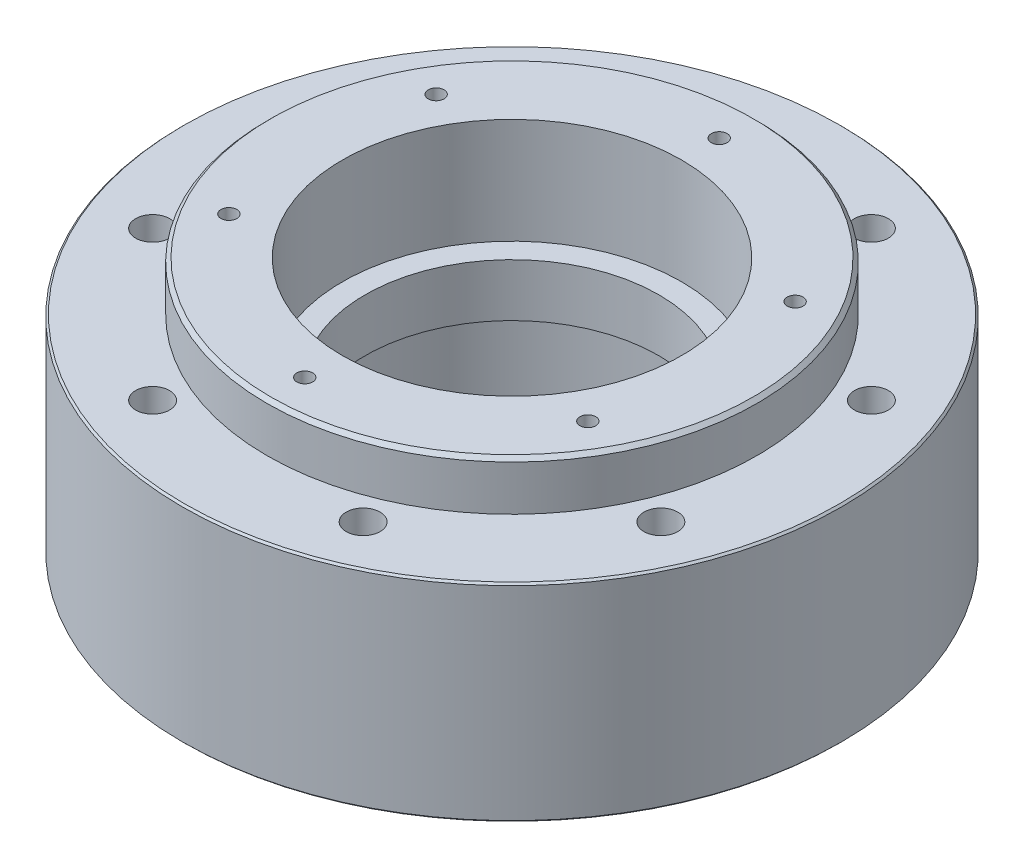
from build123d import *

# Parameters (mm, degrees)
SKETCH1_R                                          = 87.5
BOSS_EXTRUDE1_DEPTH                                = 55
SKETCH2_R                                          = 65
BOSS_EXTRUDE2_DEPTH                                = 13
SKETCH3_R                                          = 57.5
BOSS_EXTRUDE3_DEPTH                                = 5
SKETCH4_R                                          = 45
CUT_EXTRUDE1_DEPTH                                 = 31
CUT_EXTRUDE2_START                                 = -28
SKETCH5_R                                          = 45
CUT_EXTRUDE2_DEPTH                                 = 28
SKETCH6_R                                          = 39
CUT_EXTRUDE3_DEPTH                                 = 132.671940823
CHAMFER1_SIZE                                      = 1
HOLE_SIZE_BASED_ON_SOCKET_HEAD_CAP_SCR_D           = 9
HOLE_SIZE_BASED_ON_SOCKET_HEAD_CAP_SCR_CBORE_D     = 15
HOLE_SIZE_BASED_ON_SOCKET_HEAD_CAP_SCR_CBORE_DEPTH = 30
CIRPATTERN1_COUNT                                  = 8
CHAMFER2_SIZE                                      = 0.5
CIRPATTERN2_COUNT                                  = 8
CIRPATTERN3_COUNT                                  = 6


with BuildPart() as part:
    # Sketch1 → Boss-Extrude1 (new body)
    with BuildSketch(Plane(origin=(0, 0, 0), x_dir=(1, 0, 0), z_dir=(0, 1, 0))):
        with Locations(Location((0, 0, 0), (0, 0, 270))):
            Circle(SKETCH1_R)
    extrude(amount=BOSS_EXTRUDE1_DEPTH)

    # Sketch2 → Boss-Extrude2 (add)
    with BuildSketch(Plane(origin=(0, 55, 0), x_dir=(1, 0, 0), z_dir=(0, 1, 0))):
        with Locations(Location((0, 0, 0), (0, 0, 270))):
            Circle(SKETCH2_R)
    extrude(amount=BOSS_EXTRUDE2_DEPTH)

    # Sketch3 → Boss-Extrude3 (add)
    with BuildSketch(Plane.XZ):
        with Locations(Location((0, 0, 0), (0, 0, 90))):
            Circle(SKETCH3_R)
    extrude(amount=BOSS_EXTRUDE3_DEPTH)

    # Sketch4 → Cut-Extrude1 (cut)
    with BuildSketch(Plane.XZ.offset(5)):
        with Locations(Location((0, 0, 0), (0, 0, 270))):
            Circle(SKETCH4_R)
    extrude(amount=-CUT_EXTRUDE1_DEPTH, mode=Mode.SUBTRACT)

    # Sketch5 → Cut-Extrude2 (cut)
    with BuildSketch(Plane(origin=(0, 68, 0), x_dir=(1, 0, 0), z_dir=(0, 1, 0)).offset(CUT_EXTRUDE2_START)):
        with Locations(Location((0, 0, 0), (0, 0, 90))):
            Circle(SKETCH5_R)
    extrude(amount=CUT_EXTRUDE2_DEPTH, mode=Mode.SUBTRACT)

    # Sketch6 → Cut-Extrude3 (cut, through all)
    with BuildSketch(Plane(origin=(0, 40, 0), x_dir=(1, 0, 0), z_dir=(0, 1, 0))):
        with Locations(Location((0, 0, 0), (0, 0, 270))):
            Circle(SKETCH6_R)
    extrude(amount=-CUT_EXTRUDE3_DEPTH, mode=Mode.SUBTRACT)

    # Chamfer1
    chamfer1_edges = [part.edges().sort_by_distance(p)[0] for p in [
        (0, -5, -57.5),
        (0, 68, -65),
    ]]
    chamfer(chamfer1_edges, length=CHAMFER1_SIZE)

    # Hole size (% based on socket head cap screw type)1 (through all)
    with Locations(Plane(origin=(0, 0, 0), x_dir=(-1, 0, 0), z_dir=(0, -1, 0))):
        with Locations((-67.443205873, 27.935890563)):
            hole_size_based_on_socket_head_cap_scr = CounterBoreHole(HOLE_SIZE_BASED_ON_SOCKET_HEAD_CAP_SCR_D / 2, HOLE_SIZE_BASED_ON_SOCKET_HEAD_CAP_SCR_CBORE_D / 2, HOLE_SIZE_BASED_ON_SOCKET_HEAD_CAP_SCR_CBORE_DEPTH)

    # CirPattern1: Hole size (% based on socket head cap screw type)1 ×8 about axis
    cirpattern1_axis = Axis((0, 0, 0), (0, 1, 0))
    for i in range(1, CIRPATTERN1_COUNT):
        add(hole_size_based_on_socket_head_cap_scr.rotate(cirpattern1_axis, i * 360 / CIRPATTERN1_COUNT), mode=Mode.SUBTRACT)

    # Chamfer2
    chamfer2_edges = [part.edges().sort_by_distance(p)[0] for p in [
        (0, 0, -87.5),
        (0, 55, -87.5),
    ]]
    chamfer(chamfer2_edges, length=CHAMFER2_SIZE)

    # Sketch13 → M10 Tapped Hole1 (revolve, cut)
    with BuildSketch(Plane(origin=(0, 0, -67.5), x_dir=(0, 0, -1), z_dir=(1, 0, 0))):
        Polygon((0, 0), (0, 40.053657631), (4.25, 37.5), (4.25, 0), align=None)
    m10_tapped_hole1 = revolve(axis=Axis((0, -6.35, -67.5), (0, 1, 0)), mode=Mode.SUBTRACT)

    # CirPattern2: M10 Tapped Hole1 ×8 about axis
    cirpattern2_axis = Axis((0, 0, 0), (0, 1, 0))
    for i in range(1, CIRPATTERN2_COUNT):
        add(m10_tapped_hole1.rotate(cirpattern2_axis, i * 360 / CIRPATTERN2_COUNT), mode=Mode.SUBTRACT)

    # Sketch15 → M5 Tapped Hole1 (revolve, cut)
    with BuildSketch(Plane(origin=(0, 68, 55), x_dir=(0, 0, 1), z_dir=(1, 0, 0))):
        Polygon((0, 0), (0, 15.2618073), (2.1, 14), (2.1, 0), align=None)
    m5_tapped_hole1 = revolve(axis=Axis((0, 74.35, 55), (0, -1, 0)), mode=Mode.SUBTRACT)

    # CirPattern3: M5 Tapped Hole1 ×6 about axis
    cirpattern3_axis = Axis((0, 0, 0), (0, 1, 0))
    for i in range(1, CIRPATTERN3_COUNT):
        add(m5_tapped_hole1.rotate(cirpattern3_axis, i * 360 / CIRPATTERN3_COUNT), mode=Mode.SUBTRACT)


solid = part.part
